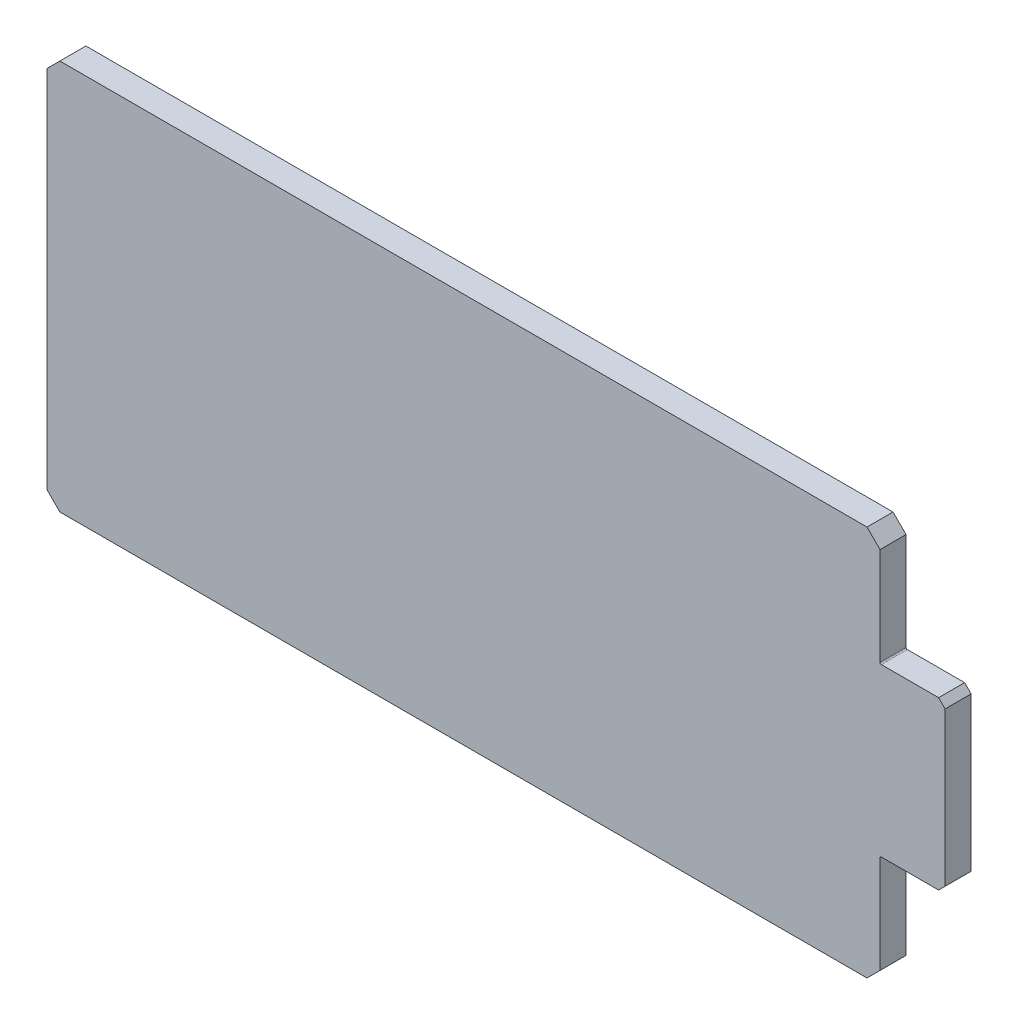
from build123d import *

# Parameters (mm, degrees)
BOSS_EXTRUDE1_DEPTH = 20
CHAMFER1_SIZE       = 10
FILLET1_R           = 1
CHAMFER2_SIZE       = 5


with BuildPart() as part:
    # Sketch1 → Boss-Extrude1 (new body)
    with BuildSketch(Plane.XY):
        Polygon((-38.770663033, -150), (-38.770663033, 150), (601.229336967, 150), (601.229336967, 64), (651.229336967, 64), (651.229336967, -64), (601.229336967, -64), (601.229336967, -150), align=None)
    extrude(amount=BOSS_EXTRUDE1_DEPTH)

    # Chamfer1
    chamfer1_edges = [part.edges().sort_by_distance(p)[0] for p in [
        (601.229336967, 150, 10),
        (601.229336967, -150, 10),
        (-38.770663033, -150, 10),
        (-38.770663033, 150, 10),
    ]]
    chamfer(chamfer1_edges, length=CHAMFER1_SIZE)

    # Fillet1
    fillet1_edges = [part.edges().sort_by_distance(p)[0] for p in [
        (601.229336967, 64, 10),
        (601.229336967, -64, 10),
    ]]
    fillet(fillet1_edges, radius=FILLET1_R)

    # Chamfer2
    chamfer2_edges = [part.edges().sort_by_distance(p)[0] for p in [
        (651.229336967, 64, 10),
        (651.229336967, -64, 10),
    ]]
    chamfer(chamfer2_edges, length=CHAMFER2_SIZE)


solid = part.part
